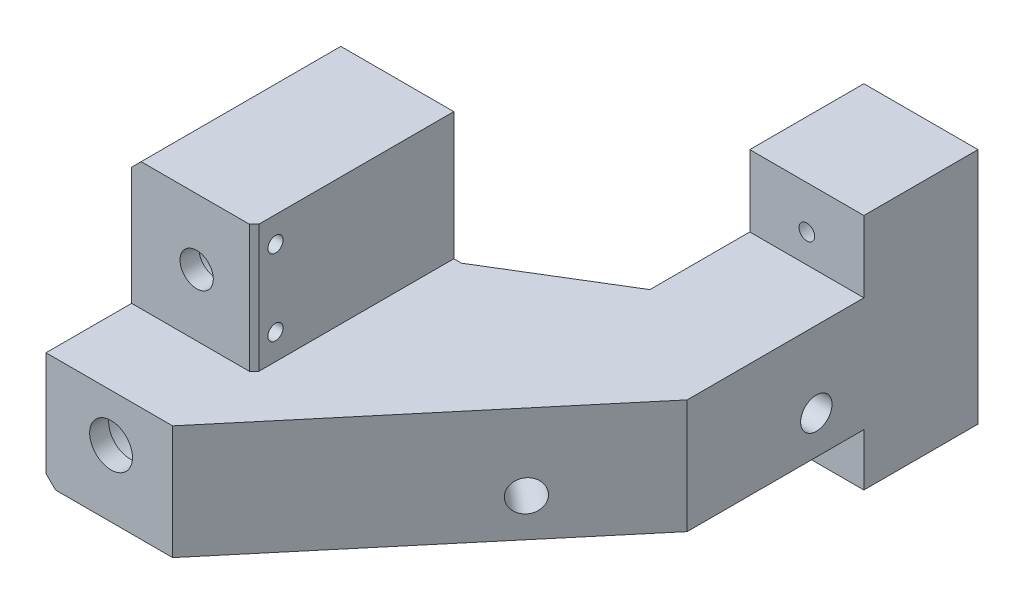
SolidWorks part; units mm, degrees
ref_plane "Front Plane" through (0, 0, 0) normal (0, 0, 1) x (1, 0, 0)
ref_plane "Top Plane" through (0, 0, 0) normal (0, 1, 0) x (1, 0, 0)
ref_plane "Right Plane" through (0, 0, 0) normal (1, 0, 0) x (0, 0, -1)
sketch "Sketch1" plane through (0, 0, 0) normal (0, 1, 0) x (1, 0, 0)
  line L0 (24, 0) -> (50, 40)
  line L1 (0, 0) -> (24, 0)
  line L2 (0, 0) -> (0, 30)
  line L3 (25, 60) -> (50, 60)
  line L4 (50, 40) -> (50, 60)
  line L5 (13.6828, 30) -> (25, 47.411)
  line L7 (0, 30) -> (13.6828, 30)
  line L8 (25, 60) -> (25, 47.411)
  dimension "D1" = 25
  dimension "D2" = 30
  dimension "D3" = 25
  dimension "D4" = 50
  dimension "D5" = 40
  dimension "D6" = 26
  dimension "D7" = 60
extrude "Boss-Extrude1" add sketch "Sketch1" along normal blind 26
sketch "Sketch2" plane through (0, 0, -60) normal (0, 0, -1) x (-1, 0, 0)
  line L1 (-50, 26) -> (-13.6828, 26)
  line L2 (-50, 26) -> (-50, 14)
  line L3 (-50, 14) -> (-13.6828, 14)
  line L4 (-13.6828, 26) -> (-13.6828, 14)
  line L5 (-50, 0) -> (-25, 0) construction
  line L6 (-13.6828, 26) -> (-13.6828, 0) construction
  dimension "D1" = 14
extrude "Cut-Extrude1" cut sketch "Sketch2" against normal blind 77
sketch "Sketch3" plane through (0, 0, 0) normal (0, 0, 1) x (1, 0, 0)
  line L0 (6.8414, 35) -> (6.8414, -49965) construction
  line L1 (0, 26) -> (13.6828, 26) construction
  line L2 (45, 7) -> (-49955, 7) construction
  line L3 (50, 14) -> (50, 0) construction
  circle A0 centre (6.8414, 7) radius 4
  circle A1 centre (6.8414, 18.5) radius 3.5
  point P4 (6.8414, 26)
  point P9 (50, 7)
  dimension "D1" = 11.5
  dimension "D2" = 8
  dimension "D3" = 7
extrude "Cut-Extrude2" cut sketch "Sketch3" against normal blind 50
sketch "Sketch4" plane through (0, 0, 0) normal (0, 0, 1) x (1, 0, 0)
  circle A0 centre (6.8414, 7) radius 2.25
  circle A1 centre (6.8414, 7) radius 4
  dimension "D1" = 4.5
  dimension "D2" = 8
extrude "Boss-Extrude2" add sketch "Sketch4" against normal blind 2
sketch "Sketch5" plane through (0, 0, 0) normal (-1, 0, 0) x (0, 0, 1)
  line L0 (-9, 12) -> (-9, 33.0008)
  line L1 (-9, 12) -> (0, 12)
  line L2 (0, 26) -> (0, 0) construction
  line L3 (-9, 33.0008) -> (0, 33.0008)
  line L4 (0, 12) -> (0, 33.0008)
  line L5 (-30, 26) -> (0, 26) construction
  dimension "D1" = 9
  dimension "D2" = 14
extrude "Cut-Extrude3" cut sketch "Sketch5" against normal blind 15
sketch "Sketch6" plane through (0, 0, -9) normal (0, 0, 1) x (1, 0, 0)
  circle A0 centre (6.8414, 18.5) radius 1.75
  circle A1 centre (6.8414, 18.5) radius 3.5
  dimension "D1" = 7
  dimension "D2" = 3.5
extrude "Boss-Extrude3" add sketch "Sketch6" against normal blind 2
sketch "Sketch10" plane through (0, 0, -60) normal (0, 0, -1) x (-1, 0, 0)
  line L0 (-50, 0) -> (-25, 0) construction
  line L1 (-38, 0) -> (-52.151, 0)
  line L2 (-38, 0) -> (-38, 19.243)
  line L3 (-38, 19.243) -> (-52.151, 19.243)
  line L4 (-52.151, 0) -> (-52.151, 19.243)
  line L5 (0, 26) -> (0, 0) construction
  dimension "D1" = 38
extrude "Cut-Extrude4" cut sketch "Sketch10" against normal blind 60
sketch "Sketch12" plane through (0, 0, -60) normal (0, 0, -1) x (-1, 0, 0)
  line L0 (-38, 0) -> (-38, 14) construction
  line L1 (-25, 0) -> (-38, 0)
  line L2 (-25, 0) -> (-25, 24)
  line L3 (-25, 24) -> (-38, 24)
  line L4 (-38, 0) -> (-38, 24)
  dimension "D1" = 24
extrude "Boss-Extrude6" add sketch "Sketch12" against normal blind 12
sketch "Sketch13" plane through (0, 24, 0) normal (0, 1, 0) x (1, 0, 0)
  line L0 (25, 60) -> (38, 60) construction
  line L1 (25, 60) -> (26, 60)
  line L2 (25, 60) -> (25, 37.5)
  line L3 (25, 37.5) -> (26, 37.5)
  line L4 (26, 60) -> (26, 37.5)
  point P5 (31.5, 60)
  dimension "D1" = 1
  dimension "D2" = 22.5
extrude "Cut-Extrude6" cut sketch "Sketch13" against normal through all
sketch "Sketch15" plane through (0, 14, 0) normal (0, 1, 0) x (1, 0, 0)
  line L0 (13.6828, 30) -> (26, 37.5)
  line L1 (26, 50.9573) -> (13.6828, 50.9573)
  line L2 (13.6828, 30) -> (13.6828, 50.9573)
  line L3 (13.3126, 0) -> (38, 0)
  line L4 (38, 29.4213) -> (38, 0)
  line L5 (26, 48) -> (26, 37.5) construction
  line L6 (38, 29.4213) -> (13.3126, 0)
  line L7 (26, 37.5) -> (26, 50.9573)
  line L8 (38, 21.5385) -> (38, 48) construction
  line L9 (15, 0) -> (0, 0) construction
  dimension "D1" = 24.6874
  dimension "D2" = 29.4213
extrude "Cut-Extrude7" cut sketch "Sketch15" against normal blind 35
sketch "Sketch18" plane through (0, 14, 0) normal (0, 1, 0) x (1, 0, 0)
  line L0 (26, 48) -> (38, 48) construction
  line L1 (38, 29.4213) -> (38, 48) construction
  line L2 (26, 48) -> (26, 37.5) construction
  line L3 (13.6828, 30) -> (26, 37.5) construction
  line L5 (38, 29.4213) -> (15, 2.011) construction
  line L6 (26, 48) -> (38, 48)
  line L7 (38, 29.4213) -> (38, 48)
  line L8 (26, 48) -> (26, 37.5)
  line L9 (13.6828, 30) -> (26, 37.5)
  line L10 (13.6828, 30) -> (13.6828, 0.4412)
  line L11 (38, 29.4213) -> (13.6828, 0.4412)
extrude "Cut-Extrude10" cut sketch "Sketch18" against normal up to surface (2 mm away) up to face at (8.6625, 12, -4.0022)
sketch "Sketch19" plane through (0, 0, -60) normal (0, 0, -1) x (-1, 0, 0)
  line L0 (-26, 0) -> (-26, 12) construction
  line L1 (-38, 0) -> (-26, 0)
  line L2 (-38, 0) -> (-38, -5.5)
  line L3 (-38, -5.5) -> (-26, -5.5)
  line L4 (-26, 0) -> (-26, -5.5)
  dimension "D1" = 5.5
extrude "Boss-Extrude7" add sketch "Sketch19" against normal up to surface (12 mm away) up to face at (32, 18, -48)
sketch "Sketch20" plane through (0, 0, -60) normal (0, 0, -1) x (-1, 0, 0)
  line L0 (-38, -5.5) -> (-38, 24) construction
  line L1 (-26, 24) -> (-38, 24)
  line L2 (-26, 24) -> (-26, 19.5)
  line L3 (-26, 19.5) -> (-38, 19.5)
  line L4 (-38, 24) -> (-38, 19.5)
  dimension "D1" = 4.5
extrude "Cut-Extrude11" cut sketch "Sketch20" against normal blind 14.6
sketch "Sketch7" plane through (0, 26, 0) normal (0, 1, 0) x (1, 0, 0)
  line L0 (13.6828, 9) -> (0, 9) construction
  line L1 (0, 30) -> (13.6828, 30)
  line L2 (0, 30) -> (0, 9)
  line L3 (0, 9) -> (13.6828, 9)
  line L4 (13.6828, 30) -> (13.6828, 9)
  line L5 (0, 9) -> (13.6828, 9) construction
extrude "Cut-Extrude9" cut sketch "Sketch7" against normal blind 0.6
sketch "Sketch21" plane through (13.6828, 0, 0) normal (1, 0, 0) x (0, 0, -1)
  line L1 (30, 12) -> (9, 12)
  line L2 (30, 12) -> (30, 25.4)
  line L3 (30, 25.4) -> (9, 25.4)
  line L4 (9, 12) -> (9, 25.4)
extrude "Cut-Extrude12" cut sketch "Sketch21" against normal blind 0.8
hole_wizard "M4 Tapped Hole1" positions "Sketch23" profile "Sketch22" tap size "M4" standard "Gb"
sketch "Sketch23" plane through (0, 0, -60) normal (0, 0, -1) x (-1, 0, 0)
  line L1 (-38, -5.5) -> (-38, 19.5) construction
  line L4 (-38, -5.5) -> (-26, -5.5) construction
  point P0 (-32, 15)
  point P2 (-32, -1)
  dimension "D1" = 16
  dimension "D2" = 6
  dimension "D3" = 4.5
cosmetic thread "Cosmetic Thread1" parameters "D1"=8, "D2"=4
cosmetic thread "Cosmetic Thread2" parameters "D1"=8, "D2"=4
sketch "Sketch22" plane through (32, 15, -60) normal (1, 0, 0) x (0, 1, 0)
  line L0 (0, 0) -> (0, 12.4914)
  line L1 (0, 12.4914) -> (1.65, 11.5)
  line L2 (1.65, 11.5) -> (1.65, 0)
  line L5 (1.65, 0) -> (0, 0)
  line L10 (0, 12.4914) -> (-1.65, 11.5) construction
  line L11 (0, -6.35) -> (0, 107.95) construction
  dimension "螺纹孔钻头直径" = 3.3
  dimension "螺纹孔钻头深度" = 11.5
  dimension "导头角度" = 118
hole_wizard "M2 Tapped Hole1" positions "Sketch25" profile "Sketch24" tap size "M2" standard "Gb"
sketch "Sketch25" plane through (12.8828, 0, 0) normal (1, 0, 0) x (0, 0, -1)
  line L0 (9, 25.4) -> (9, 12) construction
  line L1 (30, 25.4) -> (9, 25.4) construction
  point P0 (11.25, 14.7)
  point P3 (11.25, 22.7)
  dimension "D1" = 2.25
  dimension "D2" = 8
  dimension "D3" = 2.7
cosmetic thread "Cosmetic Thread3" parameters "D1"=4, "D2"=2
cosmetic thread "Cosmetic Thread4" parameters "D1"=4, "D2"=2
sketch "Sketch24" plane through (12.8828, 14.7, -11.25) normal (0, 1, 0) x (0, 0, -1)
  line L0 (0, 0) -> (0, 6.4807)
  line L1 (0, 6.4807) -> (0.8, 6)
  line L2 (0.8, 6) -> (0.8, 0)
  line L5 (0.8, 0) -> (0, 0)
  line L10 (0, 6.4807) -> (-0.8, 6) construction
  line L11 (0, -6.35) -> (0, 107.95) construction
  dimension "螺纹孔钻头直径" = 1.6
  dimension "螺纹孔钻头深度" = 6
  dimension "导头角度" = 118
hole_wizard "Ø3.0 (3) Diameter Hole1" positions "Sketch27" profile "Sketch26" hole size "Ø3.0" standard "Gb"
sketch "Sketch27" plane through (0, 0, -60) normal (0, 0, -1) x (-1, 0, 0)
  line L0 (-38, -5.5) -> (-38, 19.5) construction
  circle A0 centre (-32, -1) radius 1.65 construction
  point P0 (-32, 10)
  point P2 (-32, 4)
  dimension "D1" = 6
  dimension "D2" = 6
  dimension "D3" = 5
sketch "Sketch26" plane through (32, 10, -60) normal (1, 0, 0) x (0, 1, 0)
  line L0 (0, 0) -> (0, 8.9013)
  line L1 (0, 8.9013) -> (1.5, 8)
  line L2 (1.5, 8) -> (1.5, 0)
  line L5 (1.5, 0) -> (0, 0)
  line L10 (0, 8.9013) -> (-1.5, 8) construction
  line L11 (0, -6.35) -> (0, 107.95) construction
  dimension "孔直径" = 3
  dimension "孔深度" = 8
  dimension "导头角度" = 118
chamfer "Chamfer1" distance 0.5 angle 45 1 edges at (12.8828, 18.7, -9)
hole_wizard "M4 Tapped Hole2" positions "Sketch29" profile "Sketch28" tap size "M4" standard "Gb"
sketch "Sketch29" plane through (38, 0, 0) normal (1, 0, 0) x (0, 0, -1)
  line L0 (29.4213, 0) -> (48, 0) construction
  line L1 (48, -5.5) -> (48, 0) construction
  point P0 (43, 4)
  dimension "D1" = 4
  dimension "D2" = 5
sketch "Sketch28" plane through (38, 4, -43) normal (0, 1, 0) x (0, 0, -1)
  line L0 (0, 0) -> (0, 10.9914)
  line L1 (0, 10.9914) -> (1.65, 10)
  line L2 (1.65, 10) -> (1.65, 0)
  line L5 (1.65, 0) -> (0, 0)
  line L10 (0, 10.9914) -> (-1.65, 10) construction
  line L11 (0, -6.35) -> (0, 107.95) construction
  dimension "螺纹孔钻头直径" = 3.3
  dimension "螺纹孔钻头深度" = 10
  dimension "导头角度" = 118
cosmetic thread "Cosmetic Thread5" parameters "D1"=8, "D2"=4
hole_wizard "M4 Tapped Hole3" positions "Sketch31" profile "Sketch30" tap size "M4" standard "Gb"
sketch "Sketch31" plane through (7.8122, 0, 6.5552) normal (0.766, 0, 0.6428) x (0.6428, 0, -0.766)
  line L0 (8.5572, 0) -> (46.964, 0) construction
  line L1 (46.964, 12) -> (46.964, 0) construction
  point P0 (34.964, 4)
  dimension "D1" = 4
  dimension "D2" = 12
sketch "Sketch30" plane through (30.2865, 4, -20.2288) normal (0, 1, 0) x (0.6428, 0, -0.766)
  line L0 (0, 0) -> (0, 12.4914)
  line L1 (0, 12.4914) -> (1.65, 11.5)
  line L2 (1.65, 11.5) -> (1.65, 0)
  line L5 (1.65, 0) -> (0, 0)
  line L10 (0, 12.4914) -> (-1.65, 11.5) construction
  line L11 (0, -6.35) -> (0, 107.95) construction
  dimension "螺纹孔钻头直径" = 3.3
  dimension "螺纹孔钻头深度" = 11.5
  dimension "导头角度" = 118
cosmetic thread "Cosmetic Thread6" parameters "D1"=8, "D2"=4
chamfer "Chamfer2" distance 1 angle 45 2 edges at (0, 25.4, -19.5) (0, 0, -15)
